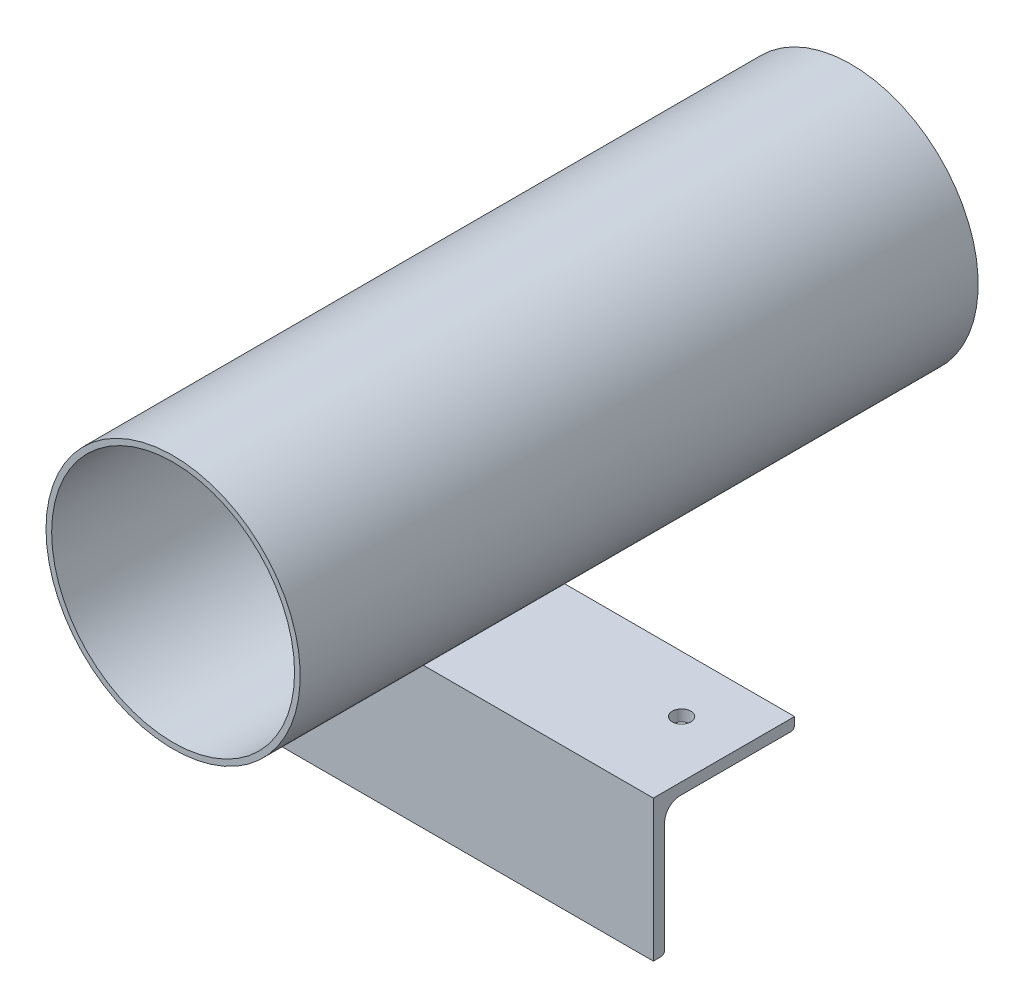
SolidWorks part; units mm, degrees
material "Q235"
ref_plane "Front Plane" through (0, 0, 0) normal (0, 0, 1) x (1, 0, 0)
ref_plane "Top Plane" through (0, 0, 0) normal (0, 1, 0) x (1, 0, 0)
ref_plane "Right Plane" through (0, 0, 0) normal (1, 0, 0) x (0, 0, -1)
sketch3d "3DSketch1"
  line L0 (0, 0, 0) -> (200, 0, 0)
  dimension "D1" = 200
other "Equal Angle Steel 5X4(1)"
ref_plane "Plane1" through (0, 0, 0) normal (1, 0, 0) x (0, 0, -1)
sketch "Sketch1" plane through (0, 0, 0) normal (1, 0, 0) x (0, 0, -1)
  line L0 (50, 0) -> (0, 0)
  line L1 (0, 0) -> (0, -50)
  line L2 (48.6667, -4) -> (9.5, -4)
  line L3 (4, -9.5) -> (4, -48.6667)
  line L4 (50, 0) -> (50, -2.6667)
  line L5 (0, -50) -> (2.6667, -50)
  arc A0 (50, -2.6667) -> (48.6667, -4) centre (48.6667, -2.6667) cw
  arc A1 (2.6667, -50) -> (4, -48.6667) centre (2.6667, -48.6667) ccw
  arc A2 (9.5, -4) -> (4, -9.5) centre (9.5, -9.5) ccw
  point P2 (25, 0)
  point P13 (0, -25)
  point P15 (0, 0)
  dimension "r1" = 1.3333
  dimension "r" = 5.5
  dimension "b" = 50
  dimension "d" = 4
sketch "Sketch3" plane through (0, 0, -50) normal (0, 0, -1) x (-1, 0, 0)
  line L0 (-100, 0) -> (-100, 45) construction
  line L1 (0, 0) -> (-200, 0) construction
  circle A0 centre (-100, 45) radius 45
  circle A1 centre (-100, 45) radius 43
  dimension "D1" = 2
  dimension "D2" = 90
  dimension "D3" = 45
extrude "Boss-Extrude1" add sketch "Sketch3" against normal blind 240 from offset 120 separate body
hole_wizard "M6 Clearance Hole1" positions "Sketch5" profile "Sketch6" hole size "M6" standard "GB"
sketch "Sketch5" plane through (0, 0, 0) normal (0, 1, 0) x (1, 0, 0)
  line L0 (200, 50) -> (0, 50) construction
  line L1 (0, 50) -> (0, 0) construction
  line L2 (200, 50) -> (200, 0) construction
  point P0 (20, 30)
  point P2 (180, 30)
  dimension "D1" = 20
  dimension "D2" = 20
  dimension "D3" = 20
sketch "Sketch6" plane through (20, 0, -30) normal (1, 0, 0) x (0, 0, 1)
  line L0 (0, 0) -> (0, 21.9828)
  line L1 (0, 21.9828) -> (3.3, 20)
  line L2 (3.3, 20) -> (3.3, 0)
  line L5 (3.3, 0) -> (0, 0)
  line L10 (0, 21.9828) -> (-3.3, 20) construction
  line L11 (0, -6.35) -> (0, 107.95) construction
  dimension "孔直径" = 6.6
  dimension "孔深度" = 20
  dimension "导头角度" = 118
